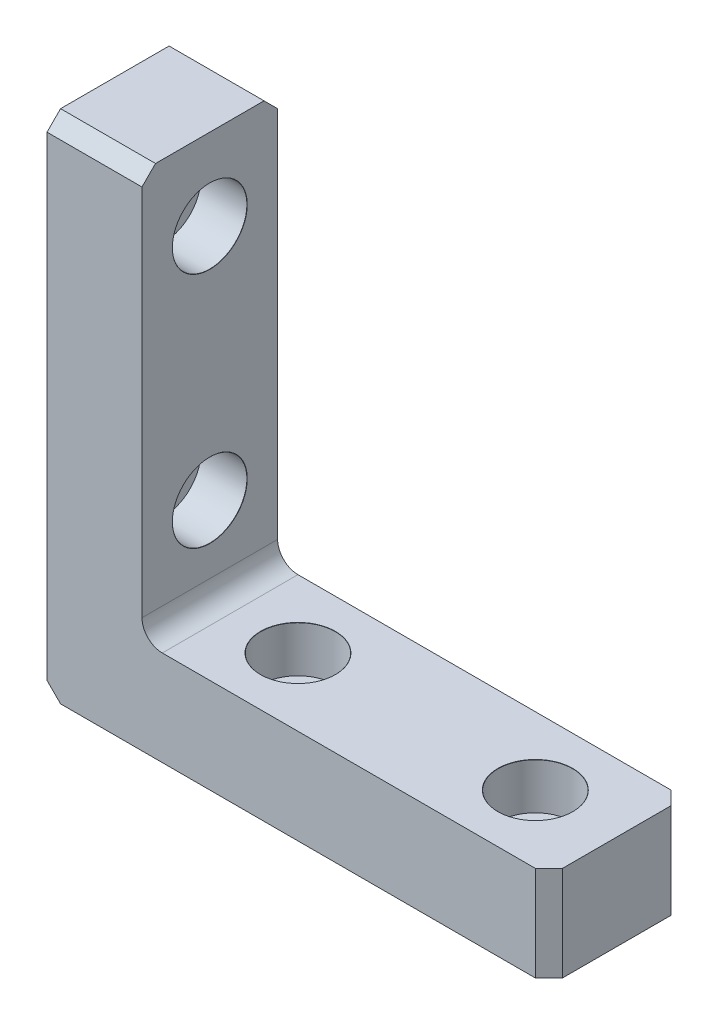
from build123d import *

# Parameters (mm, degrees)
EXTRUDE_1_DEPTH          = 10
FILLET_1_R               = 3
CHAMFER_1_SIZE           = 2
CHAMFER_2_SIZE           = 2
HOLE_WIZARD_1_AT_2_COUNT = 2
HOLE_WIZARD_1_AT_2_PITCH = 35
HOLE_WIZARD_2_AT_2_COUNT = 2
HOLE_WIZARD_2_AT_2_PITCH = 35


with BuildPart() as part:
    # 草图1 → 凸台-拉伸1 (new, symmetric)
    with BuildSketch(Plane.XY):
        Polygon((0, 0), (-74, 0), (-74, 74), (-60, 74), (-60, 14), (0, 14), align=None)
    extrude(amount=EXTRUDE_1_DEPTH, both=True)

    # 圆角1
    fillet_1_edges = [part.edges().sort_by_distance(p)[0] for p in [
        (-60, 14, 0),
    ]]
    fillet(fillet_1_edges, radius=FILLET_1_R)

    # 倒角1
    chamfer_1_edges = [part.edges().sort_by_distance(p)[0] for p in [
        (-67, 74, 10),
        (0, 7, 10),
        (-67, 74, -10),
        (0, 7, -10),
    ]]
    chamfer(chamfer_1_edges, length=CHAMFER_1_SIZE)

    # 倒角2
    chamfer_2_edges = [part.edges().sort_by_distance(p)[0] for p in [
        (-74, 0, 0),
    ]]
    chamfer(chamfer_2_edges, length=CHAMFER_2_SIZE)

    # 草图2 → 打孔尺寸(%根据)内六角圆柱头螺钉的类型1 (revolve, cut)
    with BuildSketch(Plane(origin=(-60, 62, 0), x_dir=(0, 0, -1), z_dir=(0, 1, 0))):
        Polygon((0, 0), (0, 14), (3.3, 14), (3.3, 6.8), (5.5, 6.8), (5.5, 0.025), (5.525, 0), align=None)
    hole_wizard_1 = revolve(axis=Axis((-53.65, 62, 0), (-1, 0, 0)), mode=Mode.SUBTRACT)

    # 打孔尺寸(%根据)内六角圆柱头螺钉的类型1 at 2: 打孔尺寸(%根据)内六角圆柱头螺钉的类型1 ×2
    with Locations(*[(0, -i * HOLE_WIZARD_1_AT_2_PITCH, 0) for i in range(1, HOLE_WIZARD_1_AT_2_COUNT)]):
        add(hole_wizard_1, mode=Mode.SUBTRACT)

    # 草图4 → 打孔尺寸(%根据)内六角圆柱头螺钉的类型2 (revolve, cut)
    with BuildSketch(Plane(origin=(-12, 14, 0), x_dir=(0, 0, 1), z_dir=(1, 0, 0))):
        Polygon((0, 0), (0, 14), (3.3, 14), (3.3, 6.8), (5.5, 6.8), (5.5, 0.025), (5.525, 0), align=None)
    hole_wizard_2 = revolve(axis=Axis((-12, 20.35, 0), (0, -1, 0)), mode=Mode.SUBTRACT)

    # 打孔尺寸(%根据)内六角圆柱头螺钉的类型2 at 2: 打孔尺寸(%根据)内六角圆柱头螺钉的类型2 ×2
    with Locations(*[(-i * HOLE_WIZARD_2_AT_2_PITCH, 0, 0) for i in range(1, HOLE_WIZARD_2_AT_2_COUNT)]):
        add(hole_wizard_2, mode=Mode.SUBTRACT)


solid = part.part
